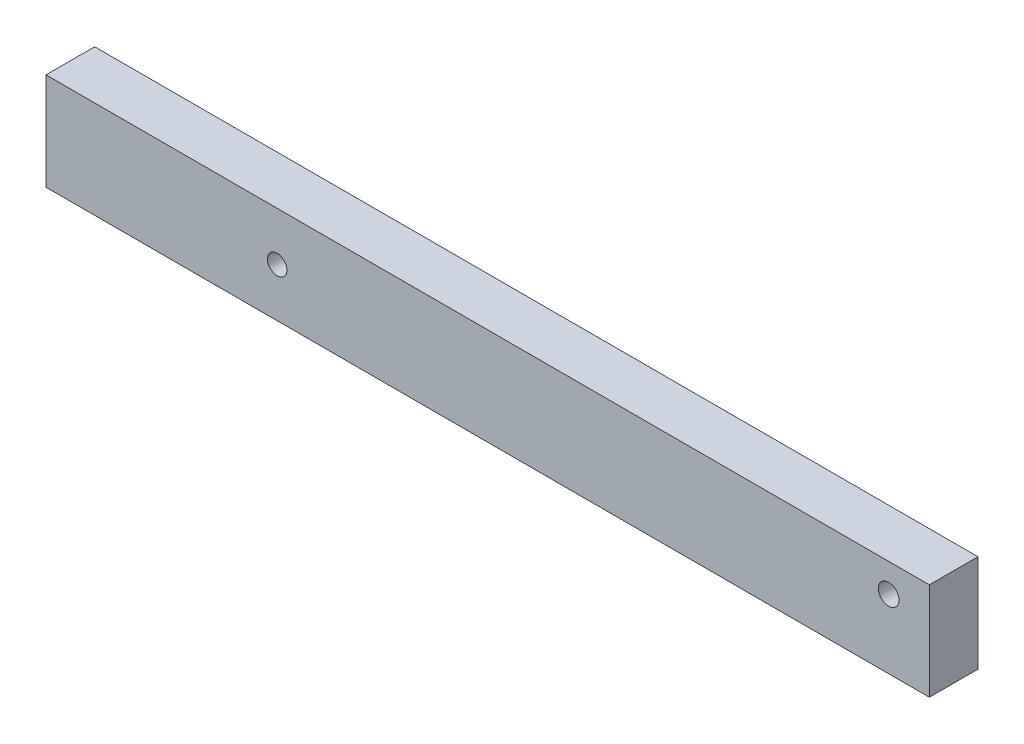
SolidWorks part; units mm, degrees
ref_plane "前视基准面" through (0, 0, 0) normal (0, 0, 1) x (1, 0, 0)
ref_plane "上视基准面" through (0, 0, 0) normal (0, 1, 0) x (1, 0, 0)
ref_plane "右视基准面" through (0, 0, 0) normal (1, 0, 0) x (0, 0, -1)
other "Configuration Table"
sketch "草图2" plane through (0, 0, 0) normal (0, 0, 1) x (1, 0, 0)
  line L1 (-200, 20) -> (200, 20)
  line L2 (-200, 20) -> (-200, -20)
  line L3 (-200, -20) -> (200, -20)
  line L4 (200, 20) -> (200, -20)
  line L5 (-200, 20) -> (200, -20) construction
  line L6 (-200, -20) -> (200, 20) construction
  circle A0 centre (180, 0) radius 4
  point P0 (0, 0)
  dimension "D3" = 8
  dimension "D1" = 400
  dimension "D2" = 40
  dimension "D4" = 20
  dimension "D5" = 20
extrude "凸台-拉伸1" add sketch "草图2" along normal blind 20
ref_plane "基准面1" through (90, 90, 0) normal (0.7071, 0.7071, 0) x (0, 0, -1)
sketch "草图3" plane through (90, 90, 0) normal (0.7071, 0.7071, 0) x (0, 0, -1)
  line L0 (-20, -127.2792) -> (0, -127.2792) construction
  circle A0 centre (-8.8759, -149.2792) radius 4
  dimension "D1" = 22
  dimension "D2" = 8
sketch "草图4" plane through (200, 0, 0) normal (1, 0, 0) x (0, 0, -1)
  line L4 (0, -20) -> (0, 20)
  line L5 (0, 20) -> (-20, 20)
  line L6 (-20, 20) -> (-20, -20)
  line L7 (-20, -20) -> (0, -20)
  line L8 (0, -20) -> (0, 20)
  line L9 (0, 20) -> (-20, 20)
  line L10 (-20, 20) -> (-20, -20)
  line L11 (-20, -20) -> (0, -20)
  dimension "D1" = 0
extrude "凸台-拉伸2" add sketch "草图4" along normal blind 248
sketch "草图5" plane through (0, 0, 20) normal (0, 0, 1) x (1, 0, 0)
  line L4 (-200, -20) -> (448, -20)
  line L5 (448, -20) -> (448, 20)
  line L6 (448, 20) -> (-200, 20)
  line L7 (-200, 20) -> (-200, -20)
  line L8 (-200, -20) -> (448, -20) construction
  line L9 (448, -20) -> (448, 20) construction
  line L10 (448, 20) -> (-200, 20) construction
  line L11 (-200, 20) -> (-200, -20) construction
  circle A1 centre (431.276, 8.288) radius 5
  point P2 (431.276, 8.288)
  dimension "D2" = 10
  dimension "D3" = 16.724
  dimension "D4" = 28.288
  dimension "D1" = 0
hole_wizard "M10 螺纹孔1" positions "草图5" profile "草图7" tap size "M10" standard "ISO" end condition through all
sketch "草图7" plane through (431.276, 8.288, 20) normal (1, 0, 0) x (0, -1, 0)
  line L0 (0, 0) -> (0, 20)
  line L1 (0, 20) -> (4.25, 20)
  line L2 (4.25, 20) -> (4.25, 0)
  line L5 (4.25, 0) -> (0, 0)
  line L11 (0, -6.35) -> (0, 107.95) construction
  dimension "通孔螺纹孔钻头直径" = 8.5
  dimension "通孔螺纹孔钻头深度" = 20
cosmetic thread "孔螺蚊线1" parameters "D2"=10
sketch "草图9" plane through (-200, 0, 0) normal (-1, 0, 0) x (0, 0, 1)
  line L4 (0, 20) -> (0, -20)
  line L5 (0, -20) -> (20, -20)
  line L6 (20, -20) -> (20, 20)
  line L7 (20, 20) -> (0, 20)
  line L8 (0, 20) -> (0, -20)
  line L9 (0, -20) -> (20, -20)
  line L10 (20, -20) -> (20, 20)
  line L11 (20, 20) -> (0, 20)
  dimension "D1" = 0
extrude "切除-拉伸2" cut sketch "草图9" against normal blind 285
